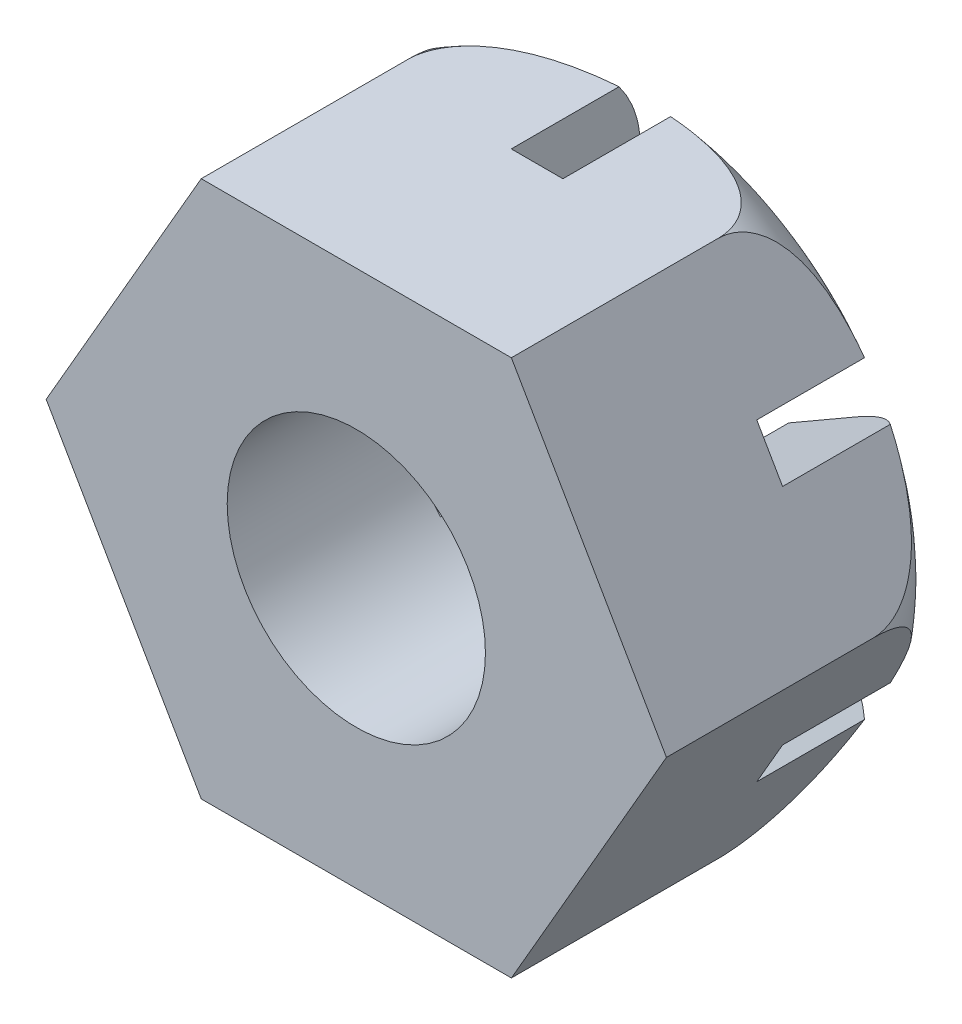
SolidWorks part; units mm, degrees
ref_plane "Front Plane" through (0, 0, 0) normal (0, 0, 1) x (1, 0, 0)
ref_plane "Top Plane" through (0, 0, 0) normal (0, 1, 0) x (1, 0, 0)
ref_plane "Right Plane" through (0, 0, 0) normal (1, 0, 0) x (0, 0, -1)
sketch "Sketch1" plane through (0, 0, 0) normal (0, 0, 1) x (1, 0, 0)
  line L1 (30.0222, -52) -> (60.0444, 0)
  line L2 (60.0444, 0) -> (30.0222, 52)
  line L3 (30.0222, 52) -> (-30.0222, 52)
  line L4 (-30.0222, 52) -> (-60.0444, 0)
  line L5 (-60.0444, 0) -> (-30.0222, -52)
  line L6 (-30.0222, -52) -> (30.0222, -52)
  circle A0 centre (0, 0) radius 52 construction
  dimension "D1" = 104
extrude "Boss-Extrude1" add sketch "Sketch1" along normal blind 60
sketch "Sketch2" plane through (0, 0, 0) normal (0, 1, 0) x (1, 0, 0)
  line L0 (0, 15.5051) -> (0, -75.6349) construction
  line L1 (-60.0444, -60) -> (-60.0444, 0) construction
  line L2 (-30.0222, 0) -> (-60.0444, 0) construction
  line L3 (-60.0444, -20) -> (-60.0444, 0)
  line L4 (-60.0444, 0) -> (-40.0444, 0)
  arc A0 (-60.0444, -20) -> (-40.0444, 0) centre (-40.0444, -20) cw
  dimension "D1" = 20
revolve "Cut-Revolve1" cut sketch "Sketch2" angle 360 about L0
sketch "Sketch3" plane through (0, 52, 0) normal (0, 1, 0) x (1, 0, 0)
  line L1 (-5, 0) -> (5, 0)
  line L2 (-5, 0) -> (-5, -25)
  line L3 (-5, -25) -> (5, -25)
  line L4 (5, 0) -> (5, -25)
  line L5 (-5, 0) -> (5, -25) construction
  line L6 (-5, -25) -> (5, 0) construction
  point P0 (0, -12.5)
  dimension "D1" = 25
  dimension "D2" = 10
extrude "Cut-Extrude1" cut sketch "Sketch3" against normal through all
pattern_circular "CirPattern1" count 6 every 60 about axis through (0, 0, 0) along (0, 0, 1) of "Cut-Extrude1"
sketch "Sketch4" plane through (0, 0, 25) normal (0, 0, -1) x (-1, 0, 0)
  circle A0 centre (0, 0) radius 25
  dimension "D1" = 50
extrude "Cut-Extrude2" cut sketch "Sketch4" along normal through all and the other way through all
